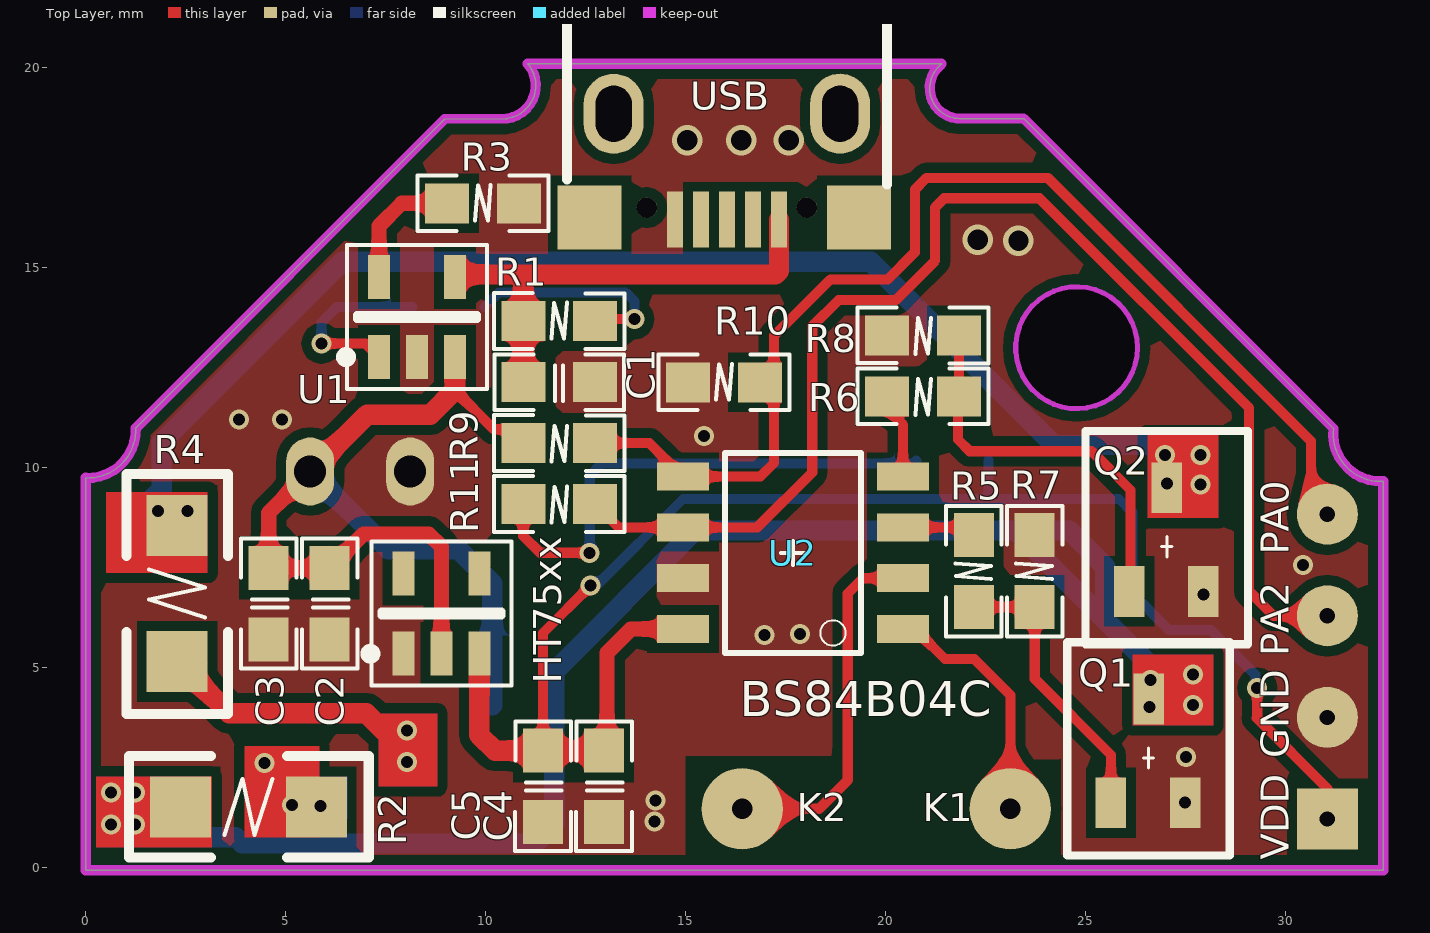
[diagram p0: Top Layer view]
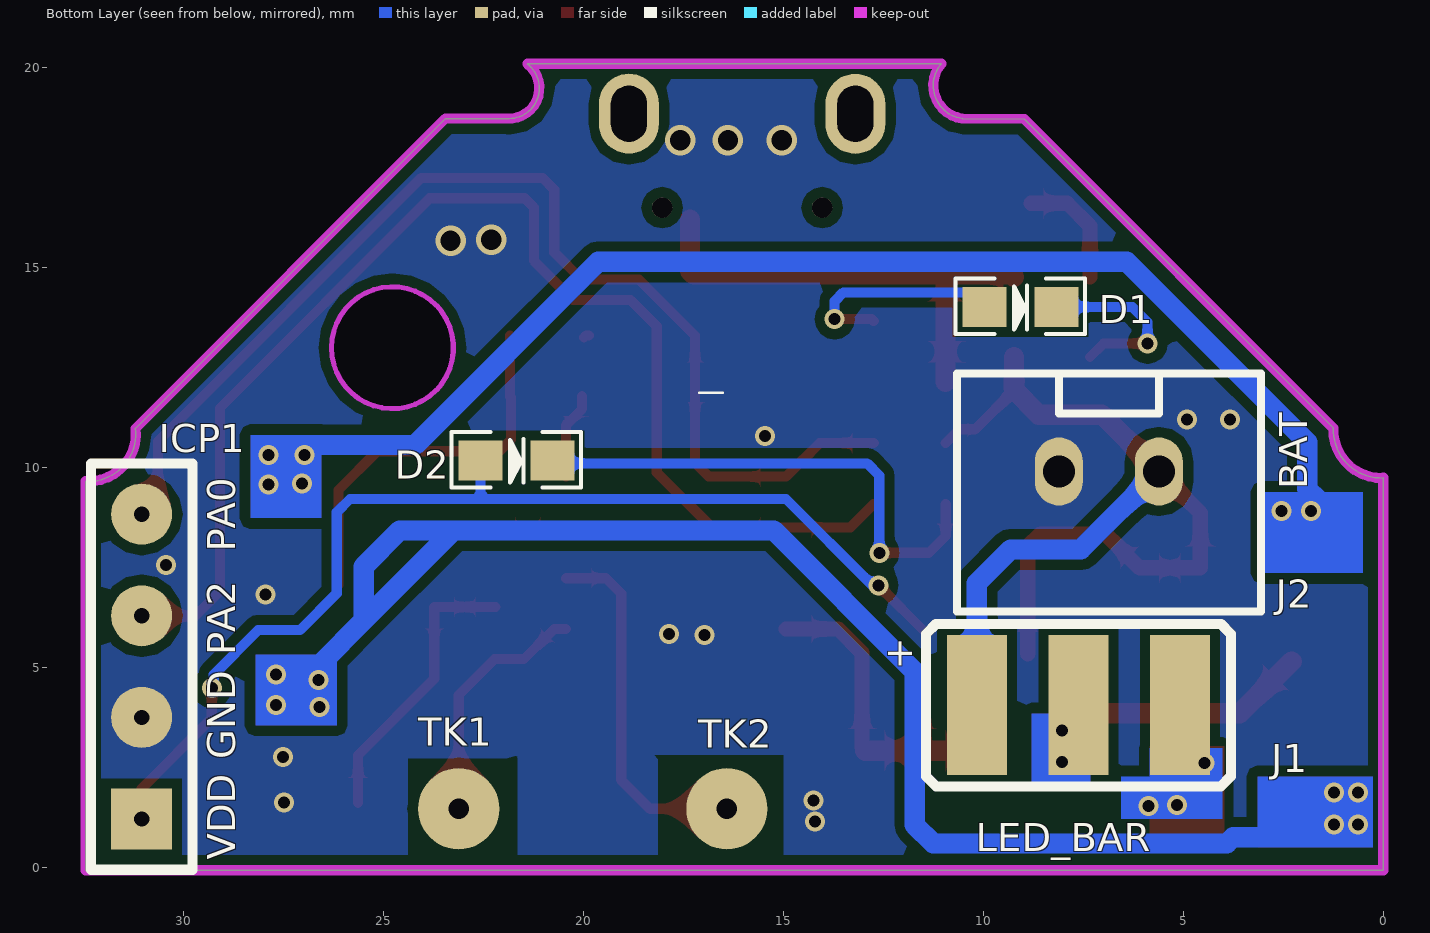
[diagram p1: Bottom Layer view, seen from below]
# Altium PCB MISC64789.PcbDoc
Units mm, origin at the board's own origin, x right, y up, seen from the top; angles counter-clockwise.
Board outline 32.44 x 20.16 mm, 2 copper layers (Top Layer, Bottom Layer); 29 components, 20 nets, 83 pads, 40 vias.

## Layer stack, top to bottom (the 12.6 mil dielectric is the usual default, probably not edited)
Top Solder: solder mask 0.0102, Solder Resist, Dk 3.5
Top Layer: signal copper 0.0356
Dielectric1: dielectric 0.32, FR-4, Dk 4.8
Bottom Layer: signal copper 0.0356
Bottom Solder: solder mask 0.0102, Solder Resist, Dk 3.5

## Board outline
0,-0.064 0,9.754 0,9.743 ccw(c0.044,10.946) 1.247,10.991 8.974,18.717 10.531,18.727 10.53,18.731 ccw(c10.414,19.558) 11.05,20.099 21.39,20.099 21.395,20.093 ccw(c21.859,19.489) 21.91,18.73 23.447,18.73 31.194,10.983 ccw(c32.365,10.839) 32.437,9.662 32.436,9.652 32.436,-0.064

## Design rules (kind name [scope] priority, off if disabled: settings)
Clearance Clearance_1 [All] p1: gap=0.254 ignorepadtopadclearanceinfootprint=FALSE except(0: Arc-Hole Track-Hole SMDPad-Hole THPad-Hole Via-Hole Fill-Hole Poly-Hole Region-Hole Text-Hole)
Clearance [All] p2: gap=0.254 ignorepadtopadclearanceinfootprint=FALSE except(0: Arc-Hole Track-Hole SMDPad-Hole THPad-Hole Via-Hole Fill-Hole Poly-Hole Region-Hole Text-Hole)
ComponentClearance [All] p1: gap=0.254 collisioncheckmode=3 verticalgap=0.254 showdistances=TRUE
ComponentClearance ComponentClearance_1 [All] p2: gap=0.254 collisioncheckmode=3 verticalgap=0.254 showdistances=TRUE
ComponentClearance ComponentClearance_2 [All] p3: gap=0.508 collisioncheckmode=3 verticalgap=0.508 showdistances=TRUE
PlaneConnect PlaneConnect_1 [All] p1: planeconnectstyle=Relief reliefexpansion=0.508 reliefentries=4 reliefconductorwidth=0.254 reliefairgap=0.254
PolygonConnect PolygonConnect_1 [All] p1: connectstyle=Direct reliefconductorwidth=0.254 reliefentries=4 polygonreliefangle="90 Angle" airgapwidth=0.254
PolygonConnect [IsVia vs IsVia] p2 off: connectstyle=Direct reliefconductorwidth=0.254 reliefentries=4 polygonreliefangle="90 Angle" airgapwidth=0.254
RoutingVias [All] p1: holewidth=0.711 width=1.27 viastyle="Through Hole" minholewidth=0.711 minwidth=1.27 maxholewidth=0.711 maxwidth=1.27
SolderMaskExpansion [All] p1: expansion=0.102 istentingtop=FALSE
Width [All] p1: maxlimit=2.54 minlimit=0.254 preferedwidth=0.254
28 further rules are at their usual default settings.

## Classes and differential pairs
component class 幾何燈: C1 C2 C3 C4 C5 D1 D2 HT75xx J1 J2 K1 K2 Q1 Q2 R1 R2 R3 R4 R5 R6 R7 R8 R9 R10 R11 U1 U2

## Components (designator, comment, footprint, x,y, rotation, side; value= is the part's Value field where it differs from the comment)
C1 "" "C 0603" 11.836,12.141 r0 top
C2 "" "C 0603" 6.096,6.604 r90 top
C3 "" "C 0603" 4.572,6.604 r90 top
C4 "" "C 0603" 12.954,2.032 r90 top
C5 "" "C 0603" 11.43,2.032 r90 top
D1 "" LED_0603 9.068,14.021 r180 bottom (schematic designator LED1)
D2 "" LED_0603 21.666,10.185 r180 bottom (schematic designator LED2)
HT75xx "HT7530" "SOT23 PIN-5" 8.89,6.35 r90 top (schematic designator U3)
ICP1 "HDR 1X4" "HDR 1x4(2.54)" 31.039,5.029 r90 bottom
J1 "HDR 1X3_2" 焊盤 5.08,4.064 r0 bottom
J2 "" "HDR 1X2 Pitch 2.5mm" 6.858,9.906 r0 bottom
K1 "SN1" KEY 23.114,1.473 r0 top (schematic designator *1)
K2 "SN1" KEY 16.408,1.473 r0 top (schematic designator *2)
Q1 "SS8050" SOT23_BJT_NPN 26.568,2.743 r0 top
Q2 "SS8050" SOT23_BJT_NPN 27.026,8.026 r0 top
R1 "1K" "R 0603" 11.836,13.665 r180 top
R2 "2R0" "R 1206" 4.064,1.524 r0 top
R3 "2K" "R 0603" 9.931,16.612 r180 top
R4 "2R0" "R 1206" 2.286,6.858 r270 top
R5 "1K" "R 0603" 22.2,7.417 r270 top
R6 "1K" "R 0603" 20.93,11.786 r0 top
R7 "1K" "R 0603" 23.724,7.417 r270 top
R8 "1K" "R 0603" 20.93,13.31 r0 top
R9 "510K" "R 0603" 11.836,10.617 r0 top
R10 "510K" "R 0603" 15.959,12.137 r180 top
R11 "1K" "R 0603" 11.836,9.093 r0 top
U1 "2KAX" "SOT23 PIN-5" 8.28,13.767 r90 top
U2 "BS84B04C" SOP8 17.678,7.874 r90 top
USB "Comment" Mcro_USB 16.027,17.526 r180 top

## Footprints (in the part's own frame and the unit in brackets; to place one, negate y for a bottom-side part, rotate by r counter-clockwise, add the part's x,y. Pads: shape width x height; smd on the part's side, far side on the other; paste and mask are expansions set on the pad)
"C 0603" [mm] "SMD 0603 2.5x1"
  rect 1.1x1 smd: 1(-0.894,0) 2(0.894,0)
  silkscreen extent -1.62,-0.7 1.62,0.69
"HDR 1X2 Pitch 2.5mm" [mm] "Header; 2 Position; Pitch 2.5"
  oval 1.2x1.7 hole 0.8: 1(-1.25,0) 2(1.25,0)
  silkscreen extent -3.8,-2.45 3.8,3.5
"HDR 1x4(2.54)" [mil]
  rect 60x60 hole 15: 1(-150,0)
  round 60 hole 15: 2(-50,0) 3(50,0) 4(150,0)
  silkscreen extent -200,-50 200,50
KEY [mil]
  round 80 hole 20: 1(0,0)
LED_0603 [mm]
  rect 1.1x1 smd: 1(-0.899,0) 2(0.899,-0.001)
  silkscreen extent -1.63,-0.68 1.61,0.71
Mcro_USB [mm]
  round 0.508 hole 0.508: 0(-2,1.025) 0(2,1.025)
  rect 0.4x1.4 smd: 1(-1.3,1.325) 2(-0.65,1.325) 3(0,1.325) 4(0.65,1.325) 5(1.3,1.325)
  rect 1.6x1.6 smd: 6(3.429,1.27) 7(-3.302,1.27)
  oval 1.5x2 hole 0.9 slot 1.4 at 90 deg: 8(-2.83,-1.325) 9(2.83,-1.324)
  silkscreen extent -4,-4.33 4,0.44
"R 0603" [mm] "SMD 0603 2.5x1"
  rect 1.1x1 smd: 1(-0.899,0) 2(0.899,0)
  silkscreen extent -1.63,-0.7 1.64,0.7
"R 1206" [mil] "SMD 1206 5x1.5"
  rect 60x60 smd: 1(-66.93,0) 2(66.93,0)
  silkscreen extent -117,-50 119,50
SOP8 [mm] "SOP8,Pitch=1.27mm,LxWxH=5.15x6.2"
  rect 0.7x1.3 smd: 1(-1.905,-2.75) 2(-0.635,-2.75) 3(0.635,-2.75) 4(1.905,-2.75) 5(1.905,2.75) 6(0.635,2.75) 7(-0.635,2.75) 8(-1.905,2.75)
  silkscreen extent -2.5,-1.7 2.5,1.7
"SOT23 PIN-5" [mm]
  rect 1.1x0.55 smd: 1(-1,0.95) 2(-1,0) 3(-1,-0.95) 4(1,-0.95) 5(1,0.95)
  silkscreen extent -1.8,-1.75 1.8,1.9
SOT23_BJT_NPN [mil]
  rect 30x50 smd: 1(36,-44) 2(-37,-44) 3(0,58)
  silkscreen extent -80,-96 80,114
焊盤 [mm]
  rect 1.5x3.5 smd: 1(0,0) 2(2.54,0) 3(5.08,0)
  silkscreen extent -1.27,-2.03 6.35,2.03

## Part data
C1 C2 C3 C4 C5: library part Cap, "?"
D1 D2: library part LED(1), "Typical INFRARED GaAs L"
HT75xx: library part H
ICP1: library part "HDR 1X4("
J1: library part HD
J2: library part "HDR 1X2(?)"
K1 K2: library part "Touch P"
Q1 Q2: library part BJT_NPN, "NPN Bipolar Transist"
R1 R2 R3 R4 R5 R6 R7 R8 R9 R10 R11: library part Resistor(1), "Resisitor"

## Free pads (board coordinates)
  round 3.048 hole 3.048: 0(24.79,13.005)

## Via types
v1: diameter 0.5, hole 0.3, Top Layer to Bottom Layer, tented both sides, 35 vias
v2: diameter 0.762, hole 0.508, Top Layer to Bottom Layer, tented both sides, 5 vias

## Nets (pads, with @x,y where several pads share a name; then routed paths per layer and width w, separated by ;. In a path a pad name is that pad's centre, name@x,y a point inside that pad or via, vN(x,y) a via of type N, cw(c..) or ccw(c..) an arc to the next point about the centre after c; other vN are vias at no path point)
3V: C4.2 C5.2 D2.1 HT75xx.3 ICP1.1 U2.8 | length 41.1
  Top Layer w0.254: C5.2 11.43,5.867 v1(12.624,7.061) ; v1(29.286,4.496) 29.286,3.759 29.273,3.746 31.039,1.981 ICP1.1
  Top Layer w0.381: C4.2 13.029,3.001 13.029,5.373 13.625,5.969 U2.8
  Top Layer w0.508: HT75xx.3 9.84,3.317 10.231,2.926 C5.2 C4.2
  Bottom Layer w0.254: v1(12.624,7.061) 12.773,7.061 14.932,9.22 22.437,9.22 ; D2.1 22.565,9.349 ; 22.764,9.218 22.696,9.218 22.694,9.22 ; 26.416,6.604 26.162,6.858 ; v1(29.286,4.496) 29.239,4.543 29.239,4.828 28.125,5.942 27.078,5.942 26.162,6.858 ; 22.437,9.22 22.694,9.22 ; 22.437,9.22 22.565,9.349 ; 22.565,9.349 22.694,9.22 ; 22.694,9.22 23.8,9.22 25.832,9.22 26.162,8.89 26.162,6.858
5V: C1.1 R1.2 U1.4 USB.1 | length 12.2
  Top Layer w0.5: U1.4 9.297,14.834 10.937,14.834 17.247,14.834 17.327,14.914 USB.1 ; 10.762,14.834 10.937,14.658 10.937,12.146 C1.1
GND: C1.2 C2.1 C3.1 C4.1 C5.1 HT75xx.1 ICP1.2 J2.2 Q1.1 Q2.1 R3.1 R7.1 R8.1 R10.2 U1.2 U2.7 USB.5 | length 0.1
  Top Layer w0.254: R8.1@19.858,13.31 19.929,13.31 R8.1@19.98,13.259
  other v1: 14.212,1.153 27.483,1.626 14.238,1.685 27.508,2.769 16.967,5.817 17.856,5.842 27.94,6.833 30.429,7.569 15.452,10.791 3.835,11.201 4.902,11.201
  other v2: 23.317,15.672 22.301,15.697 15.037,18.186 16.383,18.186 17.577,18.186
NetD1_1: D1.1 R1.1 | length 5.4
  Top Layer w0.254: R1.1 12.786,13.716 v1(13.716,13.716)
  Bottom Layer w0.254: D1.1 10.329,14.383 13.496,14.383 13.716,14.163 v1(13.716,13.716)
NetD1_2: D1.2 U1.1 | length 4.5
  Top Layer w0.254: v1(5.893,13.106) 6.991,13.106 U1.1
  Bottom Layer w0.254: v1(5.893,13.106) 5.893,13.64 6.273,14.02 D1.2
NetD2_2: D2.2 R11.1 | length 12.9
  Top Layer w0.254: R11.1 10.937,8.295 11.358,7.874 v1(12.598,7.874)
  Bottom Layer w0.254: v1(12.598,7.874) 12.598,9.804 12.903,10.109 20.692,10.109 D2.2
NetJ1_1: J1.1 R2.2 | length 0.4
  Top Layer w0.508: R2.2@5.51,1.778 R2.2
  other v1: 5.867,1.549 5.156,1.575 4.47,2.616
NetJ1_2: J1.2 R4.2 | length 6.2
  Top Layer w0.508: R4.2 3.583,3.861 7.01,3.861 7.671,3.2
  other v1: 8.026,2.642 8.026,3.429
NetK1_1: K1.1 U2.1 | length 6.2
  Top Layer w0.254: U2.1 20.728,5.969 21.479,5.218 22.214,5.218 23.114,4.318 K1.1
NetK2_1: K2.1 U2.2 | length 9.1
  Top Layer w0.254: K2.1 18.334,1.473 19.05,2.189 19.05,6.858 19.431,7.239 U2.2
NetQ1_2: Q1.2 R5.2 R7.2 | length 7.2
  Top Layer w0.254: R5.2 R7.2 23.724,4.724 25.629,2.819 Q1.2
NetQ1_3: Q1.3 R2.1 | length 37.2
  Bottom Layer w0.508: v1@1.225,1.024 1.371,1.171 1.475,1.171 1.702,1.397 2.337,0.762 3.752,0.762 3.907,0.607 11.25,0.607 11.709,1.067 11.709,4.902 15.24,8.433 23.241,8.433 ; v1@26.568,4.572 26.568,5.105 25.489,6.185 ; 23.241,8.433 25.489,6.185 ; 23.241,8.433 24.587,8.433 25.489,7.531 25.489,6.185
  other v1: 0.631,1.087 1.225,1.087 0.631,1.886 1.225,1.886 26.594,4.013 27.686,4.064 26.619,4.699 27.686,4.826
NetQ2_2: Q2.2 R6.2 R8.2 | length 9.8
  Top Layer w0.254: R8.2 R6.2 21.805,11.762 21.805,10.707 22.098,10.414 25.146,10.414 26.117,9.443 Q2.2@26.117,7.074
NetQ2_3: Q2.3 R4.1 | length 30.7
  Bottom Layer w0.508: 1.626,9.195 1.899,9.468 1.899,10.636 6.409,15.146 19.626,15.146 24.206,10.566 26.645,10.566 26.708,10.503 ; 27.559,9.119 27.864,9.423 v1(27.864,9.576)
  other v1: 1.803,8.915 2.54,8.915 27.026,9.601 26.975,10.312 27.864,10.312
NetR3_2: R3.2 U1.5 | length 3
  Top Layer w0.381: U1.5 7.33,16.043 7.899,16.612 R3.2@8.804,16.612
PA0_AD: ICP1.4 R9.2 R10.1 U2.5 | length 28.8
  Top Layer w0.254: R9.2 14.09,10.617 U2.5 16.866,9.779 17.206,10.119 17.206,12.999 17.206,13.299 18.614,14.707 20.046,14.707 20.726,15.387 20.726,16.954 21.019,17.247 24.05,17.247 30.632,10.664 30.632,9.246 ICP1.4
PA2: ICP1.3 R11.2 U2.6 | length 31.9
  Top Layer w0.254: R11.2 13.32,8.509 U2.6 16.789,8.509 18.161,9.881 18.161,13.535 18.816,14.191 20.248,14.191 21.234,15.177 21.234,16.51 21.463,16.739 23.839,16.739 29.083,11.495 29.083,6.909 29.693,6.299 ICP1.3
PWM1: R5.1 U2.3 | length 1.9
  Top Layer w0.254: U2.3@20.469,8.468 U2.3 22.006,8.509 R5.1
PWM2: R6.1 U2.4 | length 2.2
  Top Layer w0.254: R6.1 20.031,11.465 20.428,11.068 U2.4
VBAT: C2.2 C3.2 HT75xx.2 J1.3 J2.1 R9.1 U1.3 | length 26.6
  Top Layer w0.254: 9.224,11.941 10.202,10.963 10.592,10.963 R9.1
  Top Layer w0.381: J2.1 4.572,8.87 C3.2 C2.2 6.942,8.345 8.572,8.345 8.89,8.026 HT75xx.2
  Top Layer w0.508: J2.1 7.03,11.328 8.611,11.328 9.23,11.948 U1.3
  Bottom Layer w0.508: J2.1 7.557,7.957 9.315,7.957 10.16,7.112 J1.3
pads on no net: HT75xx.4 HT75xx.5 USB.0 USB.2 USB.3 USB.4 USB.6 USB.7 USB.8 USB.9

## Polygon pours and split planes (outlines as drawn)
GND on Bottom Layer "Keep-Out Layer-No Net" (solid, remove dead copper, pour order 8): -4.648,22.784 -4.47,22.606 -4.47,-2.032 36.373,-2.032 37.084,-1.321 37.541,-0.864 37.541,22.733 -3.581,22.733 -4.47,21.844
GND on Top Layer "Top Layer-No Net 1" (solid, remove dead copper, pour order 4): -1.956,22.454 34.671,22.454 34.671,-1.88 34.392,-2.159 32.233,-4.318 -1.854,-4.318 -1.854,22.352 -1.905,22.403

## Keep-outs
Keep-Out Layer:
  circle w0.127: c24.77,13 r1.524
  lines w0.254: -17.399,-68.707 -10.495,-68.707 15.041,-68.707 ; 0,9.743 ccw(c0.044,10.946) 1.247,10.991 8.974,18.717 10.531,18.727 ; 0,9.754 0,-0.064 32.436,-0.064 32.436,9.652 ; 10.53,18.731 ccw(c10.414,19.558) 11.05,20.099 21.39,20.099 ; 21.395,20.093 ccw(c21.859,19.489) 21.91,18.73 23.447,18.73 31.194,10.983 ccw(c32.365,10.839) 32.437,9.662

## Other copper
Top Layer:
  rectangle net NetQ2_3: 0.508,7.366 3.048,9.398
  rectangle net NetQ2_3: 26.543,8.738 28.321,10.82
  rectangle net NetJ1_1: 3.962,0.762 5.842,3.048
  rectangle net NetJ1_2: 7.315,2.032 8.788,3.861
  rectangle net NetQ1_3: 26.162,3.556 28.194,5.334
  rectangle net NetQ1_3: 0.254,0.508 3.15,2.286
  pour cut-out: 21.666,2.718 21.666,0.229 21.641,0.203 21.666,0.178 24.384,0.178 24.384,2.718 24.359,2.743 24.333,2.718
  pour cut-out: 14.986,0.229 18.11,0.229 18.635,0.753 18.635,2.794 15.011,2.794 14.986,2.769
  pour cut-out: 13.513,7.696 14.275,7.696 14.275,6.782 13.614,6.782 13.5,6.896 13.513,6.909
Bottom Layer:
  rectangle net NetQ2_3: 26.543,8.738 28.321,10.82
  rectangle net NetJ1_1: 4.013,1.219 5.842,2.997
  rectangle net NetJ1_2: 7.315,2.032 8.788,3.861
  rectangle net NetJ1_1: 5.842,1.219 6.553,2.286
  rectangle net NetQ2_3: 0.508,7.366 3.048,9.398
  rectangle net NetQ1_3: 26.162,3.556 28.194,5.334
  rectangle net NetQ1_3: 0.254,0.508 3.15,2.286
  pour cut-out: 21.692,2.794 21.641,2.743 21.641,0.203 24.409,0.203 24.384,0.229 24.384,2.743 21.666,2.743 21.641,2.769
  pour cut-out: 18.237,2.819 18.136,2.718 18.136,0.152 15.037,0.152 14.935,0.254 14.986,0.305 14.986,2.819

## Silkscreen, mask and mechanical layers (free items; w line width, h text height)
Top Overlay:
  text "PA0" at 30.074,7.824 h0.7 r90
  text "PA2" at 30.074,5.284 h0.7 r90
  text "BS84B04C" at 16.351,3.502 h1.5
  text "GND" at 30.074,2.744 h0.7 r90
  text "VDD" at 30.074,0.204 h0.7 r90
Bottom Overlay:
  lines w0.064: 16.51,11.874 17.094,11.874
  text "BAT" at 1.899,9.468 h0.7 r270
  text "PA0" at 28.702,7.899 h0.7 r270
  text "PA2" at 28.702,5.309 h0.7 r270
  text "+" at 12.37,4.953 h0.7 r90
  text "TK1" at 24.13,3.048 h0.7
  text "TK2" at 17.12,2.997 h0.7
  text "GND" at 28.702,2.718 h0.7 r270
  text "LED_BAR" at 10.185,0.406 h0.7
  text "VDD" at 28.702,0.203 h0.7 r270
Mechanical 15:
  lines w0.003: 16.195,10.024 16.246,10.075